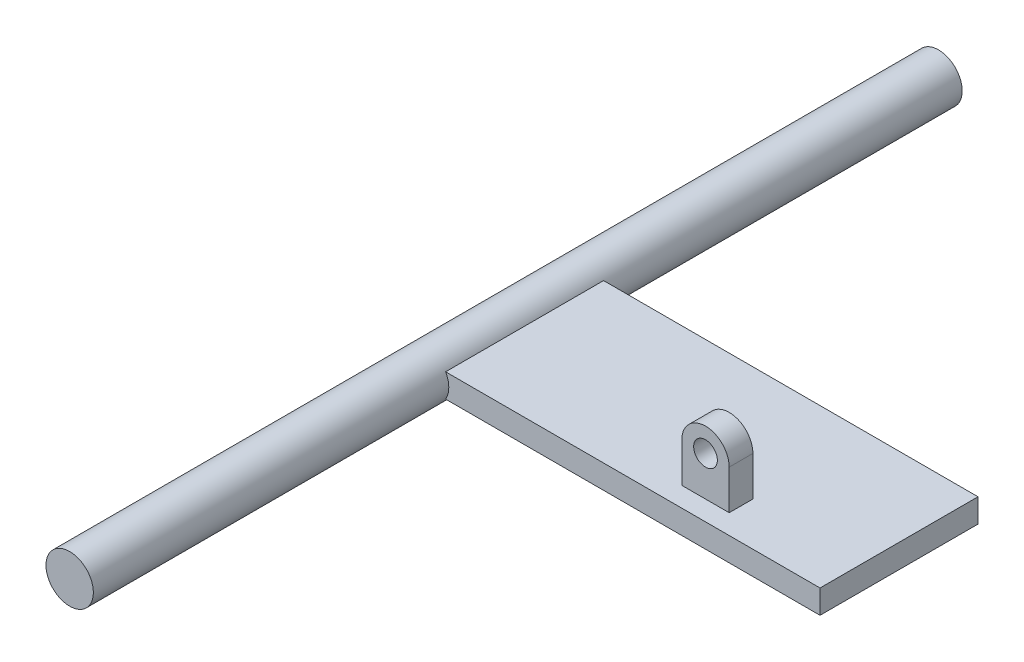
SolidWorks part; units mm, degrees
ref_plane "Front Plane" through (0, 0, 0) normal (0, 0, 1) x (1, 0, 0)
ref_plane "Top Plane" through (0, 0, 0) normal (0, 1, 0) x (1, 0, 0)
ref_plane "Right Plane" through (0, 0, 0) normal (1, 0, 0) x (0, 0, -1)
other "Configuration Table"
sketch "Sketch1" plane through (0, 0, 0) normal (0, 0, 1) x (1, 0, 0)
  circle A0 centre (0, 0) radius 3
  dimension "D1" = 6
extrude "Boss-Extrude1" add sketch "Sketch1" along normal mid plane 110
sketch "Sketch2" plane through (0, 0, 0) normal (0, 0, 1) x (1, 0, 0)
  line L1 (50, 1.5) -> (0, 1.5)
  line L2 (50, 1.5) -> (50, -1.5)
  line L3 (50, -1.5) -> (0, -1.5)
  line L4 (0, 1.5) -> (0, -1.5)
  line L5 (25, -1.5) -> (25, 1.5) construction
  line L6 (50, 0) -> (0, 0) construction
  point P0 (25, 0)
  dimension "D1" = 50
  dimension "D2" = 3
extrude "Boss-Extrude2" add sketch "Sketch2" along normal mid plane 20
ref_plane "Plane1" through (0, 0, 7.5) normal (0, 0, 1) x (1, 0, 0)
sketch "Sketch3" plane through (0, 0, 7.5) normal (0, 0, 1) x (1, 0, 0)
  line L0 (30, 6.5) -> (30, 1.5)
  line L1 (50, 1.5) -> (2.5981, 1.5) construction
  line L2 (30, 1.5) -> (36, 1.5)
  line L3 (36, 1.5) -> (36, 6.5)
  circle A0 centre (33, 6.5) radius 3
  circle A1 centre (33, 6.5) radius 1.5
  dimension "D1" = 3
  dimension "D2" = 6
  dimension "D3" = 5
  dimension "D4" = 30
extrude "Boss-Extrude3" add sketch "Sketch3" against normal blind 3 contours A0 A1 | A0 L0 L2 L3
